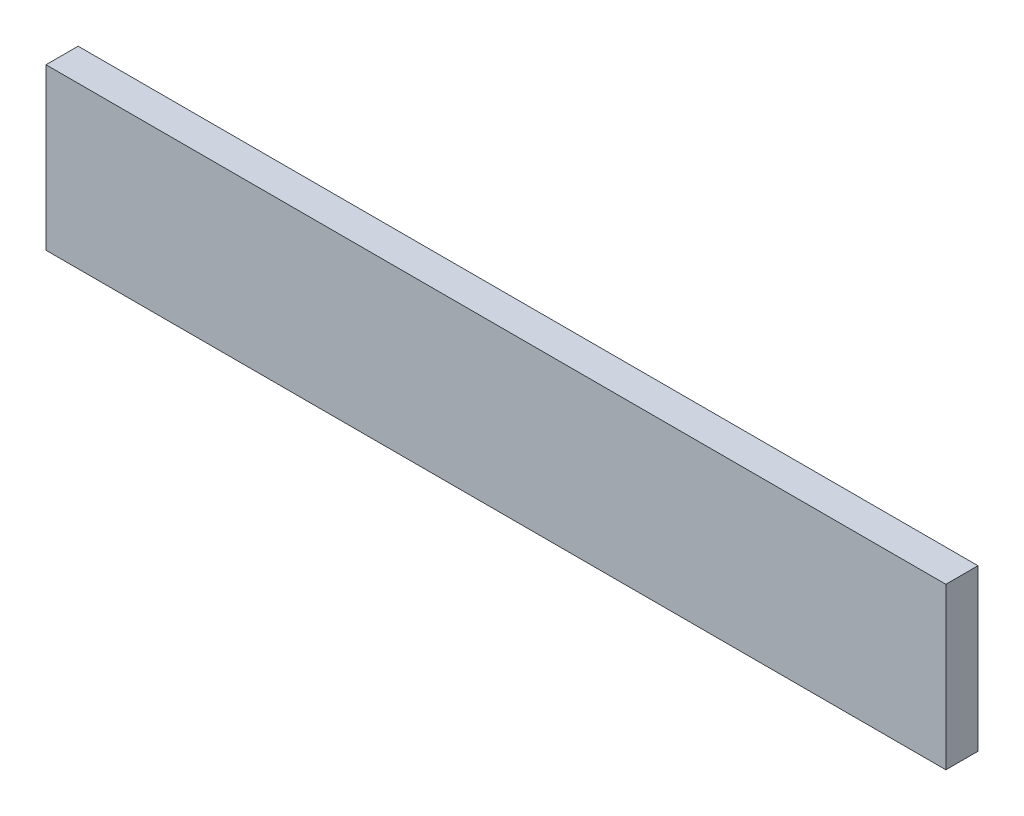
SolidWorks part; units mm, degrees
ref_plane "前视基准面" through (0, 0, 0) normal (0, 0, 1) x (1, 0, 0)
ref_plane "上视基准面" through (0, 0, 0) normal (0, 1, 0) x (1, 0, 0)
ref_plane "右视基准面" through (0, 0, 0) normal (1, 0, 0) x (0, 0, -1)
sketch "草图1" plane through (0, 0, 0) normal (0, 0, 1) x (1, 0, 0)
  line L1 (-70, -12.5) -> (70, -12.5)
  line L2 (-70, -12.5) -> (-70, 12.5)
  line L3 (-70, 12.5) -> (70, 12.5)
  line L4 (70, -12.5) -> (70, 12.5)
  line L5 (-70, -12.5) -> (70, 12.5) construction
  line L6 (-70, 12.5) -> (70, -12.5) construction
  point P0 (0, 0)
  dimension "D1" = 140
  dimension "D2" = 25
extrude "凸台-拉伸1" add sketch "草图1" along normal blind 5
